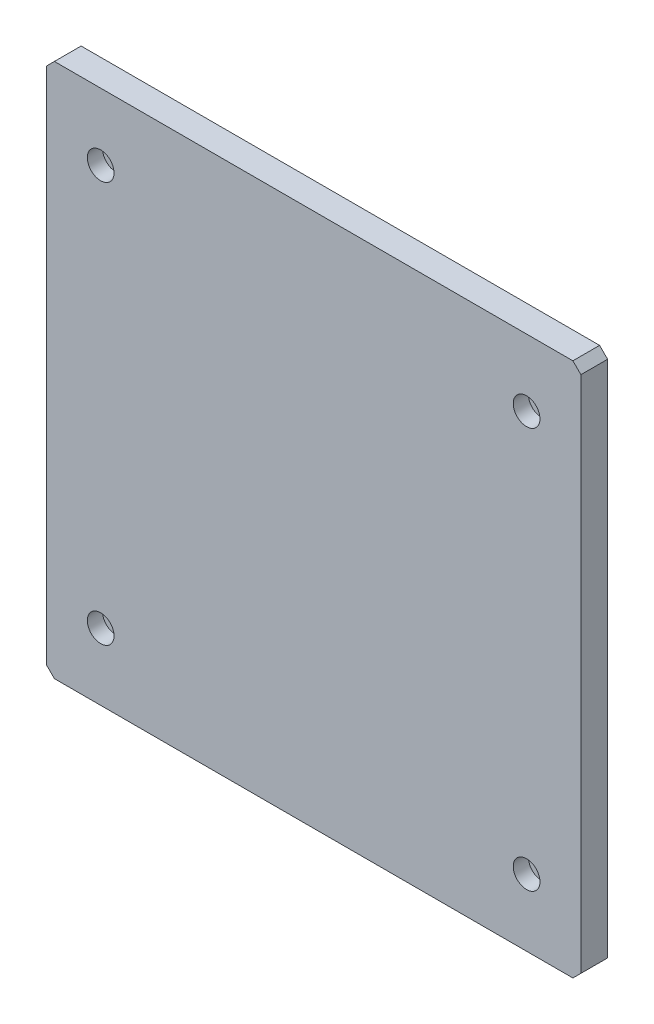
SolidWorks part; units mm, degrees
ref_plane "Front Plane" through (0, 0, 0) normal (0, 0, 1) x (1, 0, 0)
ref_plane "Top Plane" through (0, 0, 0) normal (0, 1, 0) x (1, 0, 0)
ref_plane "Right Plane" through (0, 0, 0) normal (1, 0, 0) x (0, 0, -1)
sketch "Sketch1" plane through (0, 0, 0) normal (0, 0, 1) x (1, 0, 0)
  line L1 (-100, -100) -> (100, -100)
  line L2 (-100, -100) -> (-100, 100)
  line L3 (-100, 100) -> (100, 100)
  line L4 (100, -100) -> (100, 100)
  line L5 (-100, -100) -> (100, 100) construction
  line L6 (-100, 100) -> (100, -100) construction
  point P0 (0, 0)
  dimension "D1" = 200
  dimension "D2" = 200
extrude "Boss-Extrude1" add sketch "Sketch1" along normal blind 10
hole_wizard "CBORE for M5 Hexagon socket head cap screws1" positions "Sketch2" profile "Sketch3" counterbore size "M5" standard "GB"
sketch "Sketch2" plane through (0, 0, 10) normal (0, 0, 1) x (1, 0, 0)
  point P0 (-79.6802, 75)
  point P3 (79.6802, 75)
  point P6 (79.6802, -75)
  point P9 (-79.6802, -75)
sketch "Sketch3" plane through (-79.6802, 75, 10) normal (1, 0, 0) x (0, -1, 0)
  line L0 (0, 0) -> (0, 38.5524)
  line L1 (0, 38.5524) -> (2.75, 36.9)
  line L2 (2.75, 36.9) -> (2.75, 5.7)
  line L3 (2.75, 5.7) -> (5, 5.7)
  line L4 (5, 5.7) -> (5, 0)
  line L5 (5, 0) -> (0, 0)
  line L10 (0, 38.5524) -> (-2.75, 36.9) construction
  line L11 (0, -6.35) -> (0, 107.95) construction
  dimension "孔直径" = 5.5
  dimension "孔深度" = 36.9
  dimension "柱形沉头孔直径" = 10
  dimension "柱形沉头孔深度" = 5.7
  dimension "导头角度" = 118
chamfer "Chamfer1" distance 3 angle 45 4 edges at (-100, 100, 5) (100, 100, 5) (-100, -100, 5) (100, -100, 5)
equation "\"1\"= \"代号代号\""
equation "\"2\"= \"名称代号\""
